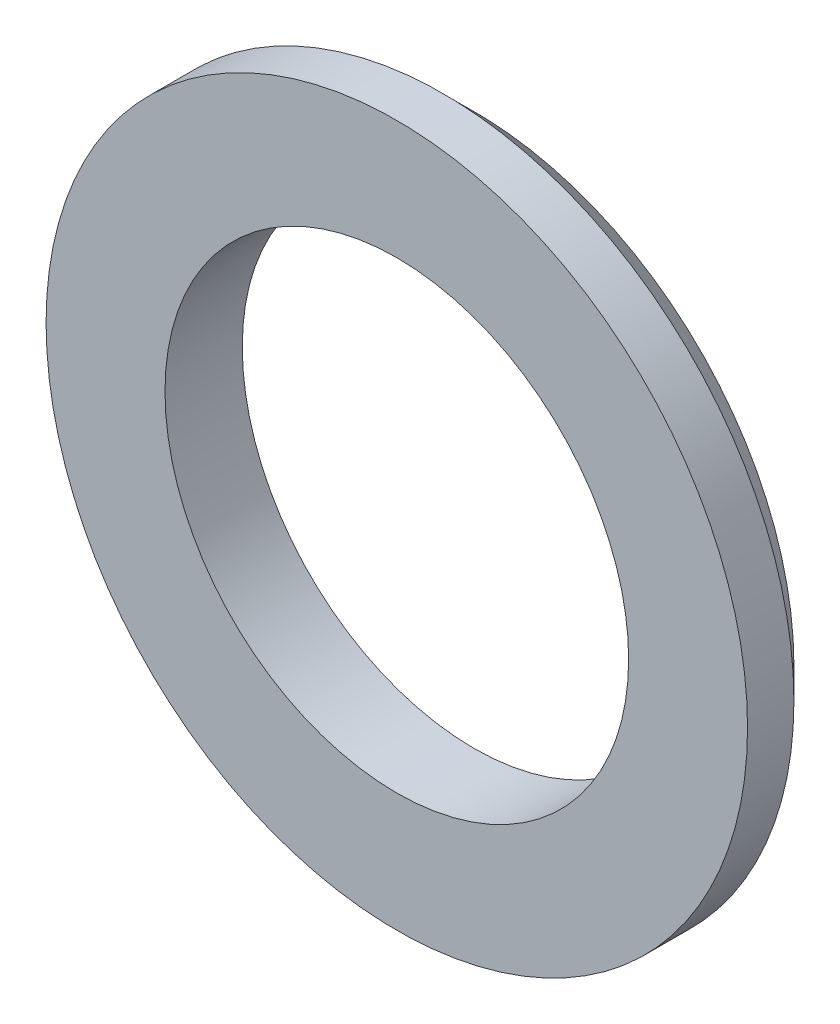
from build123d import *

# Parameters (mm, degrees)
SKETCH2_R           = 22.693719158
SKETCH2_R_2         = 15
BOSS_EXTRUDE1_DEPTH = 5
CHAMFER1_SIZE       = 2


with BuildPart() as part:
    # Sketch2 → Boss-Extrude1 (new body)
    with BuildSketch(Plane.XY):
        with Locations((70, -13)):
            Circle(SKETCH2_R)
        with Locations((70, -13)):
            Circle(SKETCH2_R_2, mode=Mode.SUBTRACT)
    extrude(amount=BOSS_EXTRUDE1_DEPTH)

    # Chamfer1
    chamfer1_edges = [part.edges().sort_by_distance(p)[0] for p in [
        (47.306280842, -13, 0),
    ]]
    chamfer(chamfer1_edges, length=CHAMFER1_SIZE)


solid = part.part
